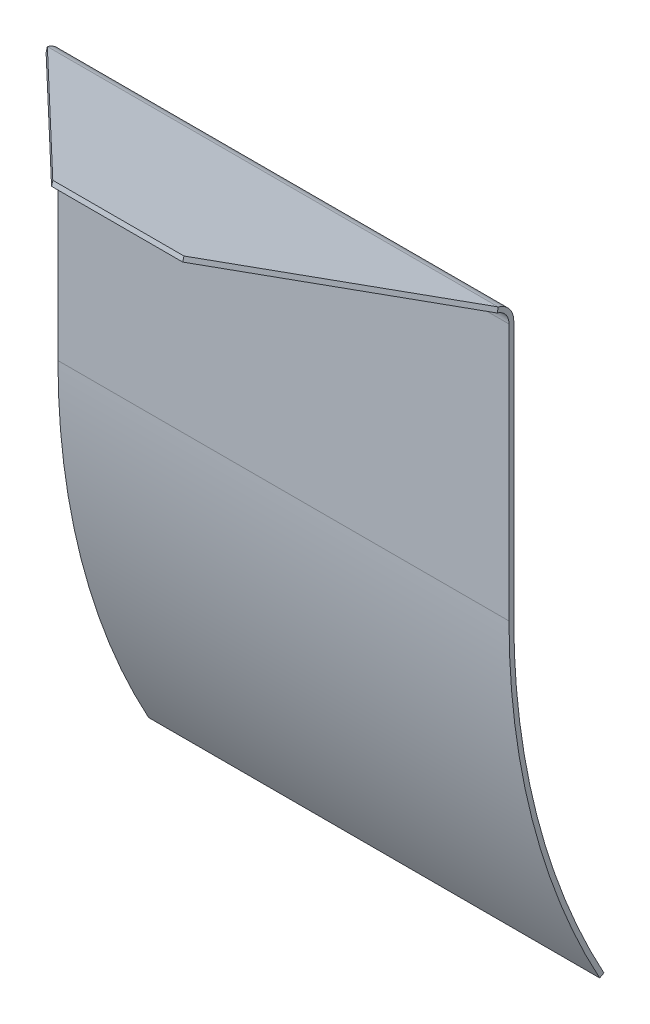
from build123d import *

# Parameters (mm, degrees)
BOSS_EXTRUDE1_DEPTH = 70.5
CHAMFER1_SIZE       = 50


with BuildPart() as part:
    # Sketch1 → Boss-Extrude1 (new, symmetric)
    with BuildSketch(Plane(origin=(0, 0, 0), x_dir=(0, 0, -1), z_dir=(1, 0, 0))):
        with BuildLine():
            ThreePointArc((-230.8, 80.4), (-231.833233299, 83.443807145), (-234.505904774, 85.229629131))
            Line((-234.505904774, 85.229629131), (-282.802196089, 98.170581387))
            Line((-282.802196089, 98.170581387), (-282.413967521, 99.619470126))
            Line((-282.413967521, 99.619470126), (-234.117676207, 86.678517871))
            ThreePointArc((-234.117676207, 86.678517871), (-230.643203288, 84.356949289), (-229.3, 80.4))
            Line((-229.3, 80.4), (-229.3, 0))
            ThreePointArc((-229.3, 0), (-222.145797616, -56.830754012), (-201.129615338, -110.115247964))
            Line((-201.129615338, -110.115247964), (-202.445334583, -110.83558321))
            ThreePointArc((-202.445334583, -110.83558321), (-223.598997339, -57.202520828), (-230.8, 0))
            Line((-230.8, 0), (-230.8, 80.4))
        make_face()
    extrude(amount=BOSS_EXTRUDE1_DEPTH, both=True)

    # Chamfer1
    chamfer1_edges = [part.edges().sort_by_distance(p)[0] for p in [
        (-70.5, 98.895025756, 282.608081805),
        (70.5, 98.895025756, 282.608081805),
    ]]
    chamfer(chamfer1_edges, length=CHAMFER1_SIZE)


solid = part.part
